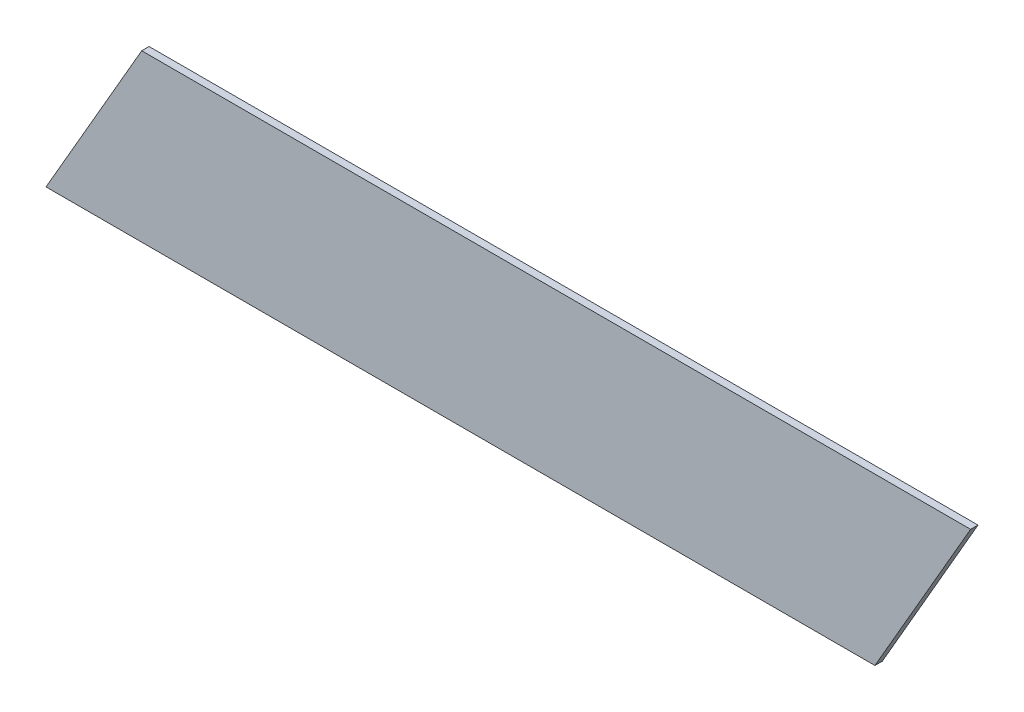
from build123d import *

# Parameters (mm, degrees)
BOSS_EXTRUDE1_DEPTH = 0.4


with BuildPart() as part:
    # Sketch1 → Boss-Extrude1 (new body)
    with BuildSketch(Plane.XY):
        Polygon((0, 0), (45, 0), (50.196152423, 9), (5.196152423, 9), align=None)
    extrude(amount=BOSS_EXTRUDE1_DEPTH)


solid = part.part
